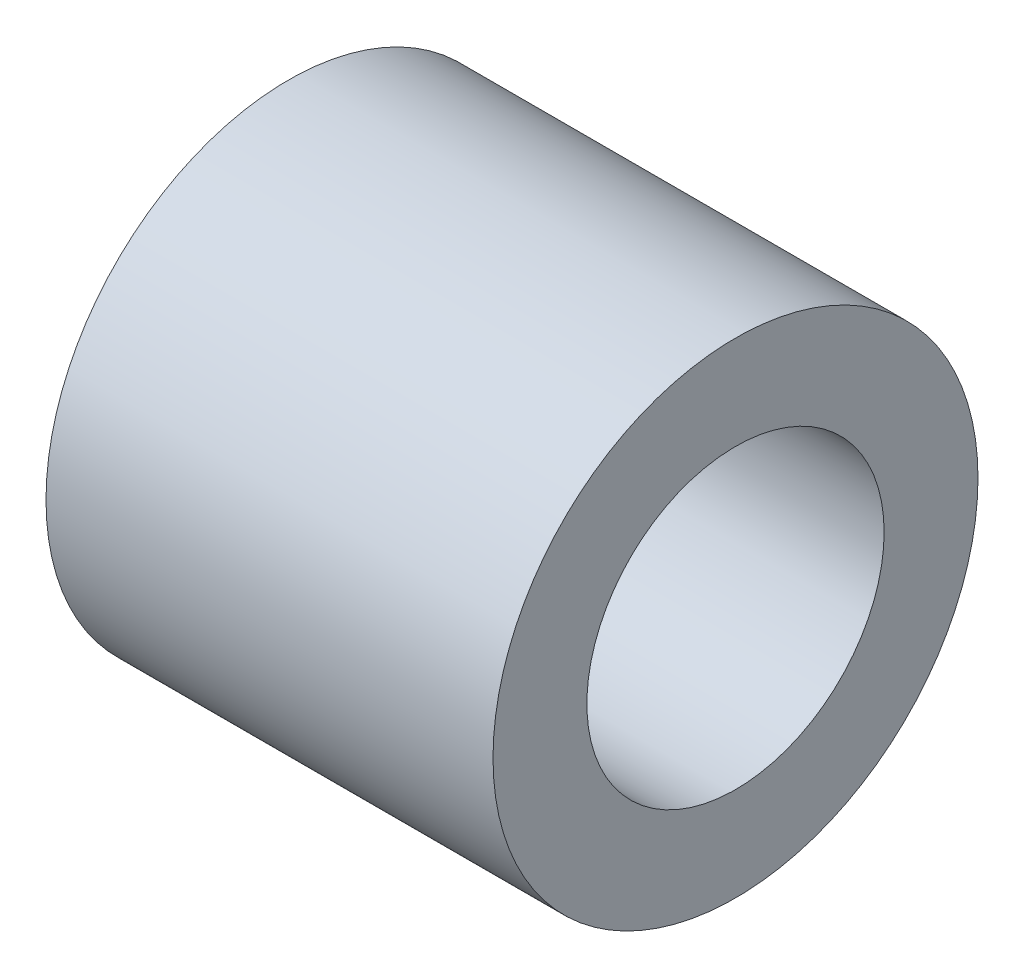
SolidWorks part; units mm, degrees
material "STKM13A"
ref_plane "Front Plane" through (0, 0, 0) normal (0, 0, 1) x (1, 0, 0)
ref_plane "Top Plane" through (0, 0, 0) normal (0, 1, 0) x (1, 0, 0)
ref_plane "Right Plane" through (0, 0, 0) normal (1, 0, 0) x (0, 0, -1)
sketch "Sketch1" plane through (0, 0, 0) normal (1, 0, 0) x (0, 0, -1)
  circle A0 centre (0, 0) radius 10.85
  circle A1 centre (0, 0) radius 6.65
  dimension "D1" = 21.7
  dimension "D2" = 4.2
extrude "Boss-Extrude1" add sketch "Sketch1" along normal blind 20
